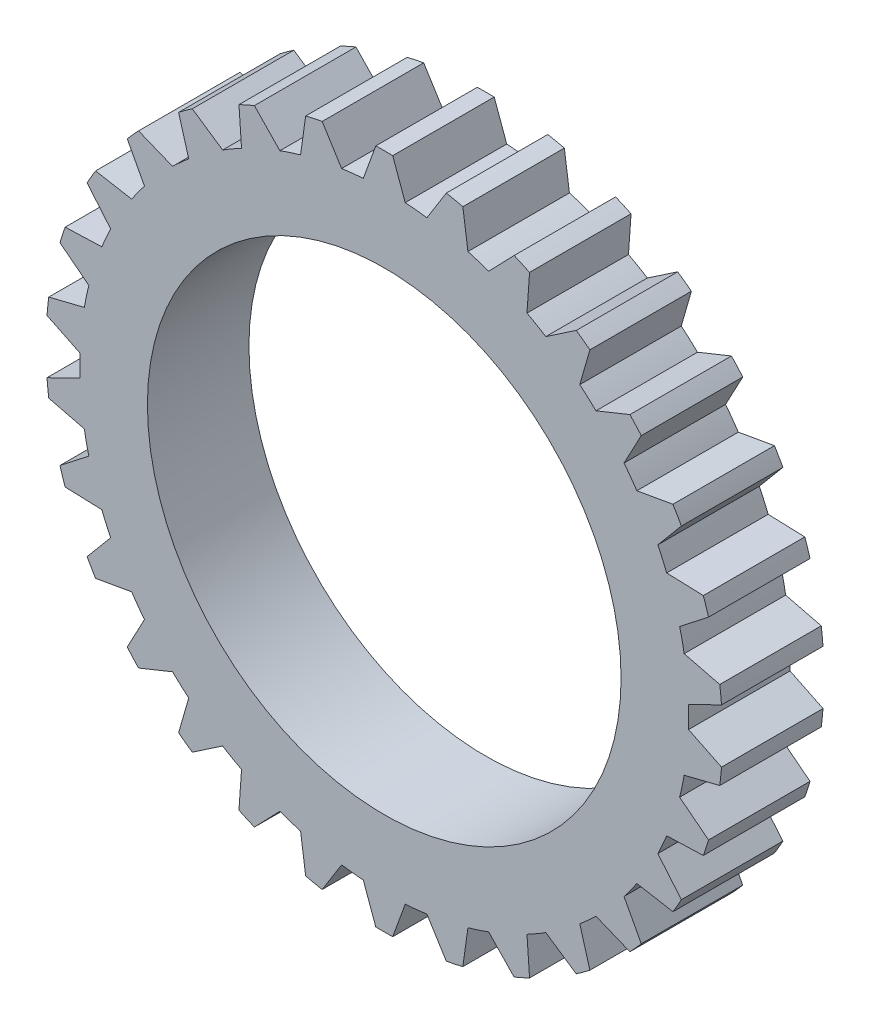
from build123d import *

# Parameters (mm, degrees)
SKETCH1_R           = 70
BOSS_EXTRUDE1_DEPTH = 30


with BuildPart() as part:
    # Sketch1 → Boss-Extrude1 (new body)
    with BuildSketch(Plane.XY):
        with BuildLine():
            Line((-2.5, 99.968745116), (-6.2, 89.786190475))
            ThreePointArc((-6.2, 89.786190475), (-9.407561694, 89.506970583), (-12.603083549, 89.113199275))
            Line((-12.603083549, 89.113199275), (-18.339301824, 98.30396741))
            ThreePointArc((-18.339301824, 98.30396741), (-20.791169082, 97.814760073), (-23.230039828, 97.264408956))
            Line((-23.230039828, 97.264408956), (-24.732113798, 86.535094309))
            ThreePointArc((-24.732113798, 86.535094309), (-27.811529494, 85.595086467), (-30.855351871, 84.545533654))
            Line((-30.855351871, 84.545533654), (-38.377088157, 92.342834614))
            ThreePointArc((-38.377088157, 92.342834614), (-40.673664308, 91.354545764), (-42.944815445, 90.309151399))
            Line((-42.944815445, 90.309151399), (-42.183315546, 79.50199928))
            ThreePointArc((-42.183315546, 79.50199928), (-45, 77.942286341), (-47.759093256, 76.282822519))
            Line((-47.759093256, 76.282822519), (-56.737611583, 82.345876836))
            ThreePointArc((-56.737611583, 82.345876836), (-58.778525229, 80.901699437), (-60.782696555, 79.406950574))
            Line((-60.782696555, 79.406950574), (-57.790903986, 68.99428539))
            ThreePointArc((-57.790903986, 68.99428539), (-60.221754572, 66.883034293), (-62.575533091, 64.686185993))
            Line((-62.575533091, 64.686185993), (-72.618429126, 68.7500091))
            ThreePointArc((-72.618429126, 68.7500091), (-74.314482548, 66.913060636), (-75.964082158, 65.034284972))
            Line((-75.964082158, 65.034284972), (-70.87275261, 55.471190157))
            ThreePointArc((-70.87275261, 55.471190157), (-72.811529494, 52.900672706), (-74.65712186, 50.262452741))
            Line((-74.65712186, 50.262452741), (-85.325472855, 52.149436067))
            ThreePointArc((-85.325472855, 52.149436067), (-86.602540378, 50), (-87.825472855, 47.819309048))
            Line((-87.825472855, 47.819309048), (-80.85712186, 39.523737734))
            ThreePointArc((-80.85712186, 39.523737734), (-82.219091188, 36.606297877), (-83.475836159, 33.642009118))
            Line((-83.475836159, 33.642009118), (-94.303383982, 33.269682438))
            ThreePointArc((-94.303383982, 33.269682438), (-95.10565163, 30.901699437), (-95.848468954, 28.514399856))
            Line((-95.848468954, 28.514399856), (-87.30764689, 21.848908316))
            ThreePointArc((-87.30764689, 21.848908316), (-88.033284066, 18.712052174), (-88.646255857, 15.551248264))
            Line((-88.646255857, 15.551248264), (-99.159784712, 12.93588404))
            ThreePointArc((-99.159784712, 12.93588404), (-99.452189537, 10.452846327), (-99.682427028, 7.963274563))
            Line((-99.682427028, 7.963274563), (-89.942408801, 3.219176762))
            ThreePointArc((-89.942408801, 3.219176762), (-90, 0), (-89.942408801, -3.219176762))
            Line((-89.942408801, -3.219176762), (-99.682427028, -7.963274563))
            ThreePointArc((-99.682427028, -7.963274563), (-99.452189537, -10.452846327), (-99.159784712, -12.93588404))
            Line((-99.159784712, -12.93588404), (-88.646255857, -15.551248264))
            ThreePointArc((-88.646255857, -15.551248264), (-88.033284066, -18.712052174), (-87.30764689, -21.848908316))
            Line((-87.30764689, -21.848908316), (-95.848468954, -28.514399856))
            ThreePointArc((-95.848468954, -28.514399856), (-95.10565163, -30.901699437), (-94.303383982, -33.269682438))
            Line((-94.303383982, -33.269682438), (-83.475836159, -33.642009118))
            ThreePointArc((-83.475836159, -33.642009118), (-82.219091188, -36.606297877), (-80.85712186, -39.523737734))
            Line((-80.85712186, -39.523737734), (-87.825472855, -47.819309048))
            ThreePointArc((-87.825472855, -47.819309048), (-86.602540378, -50), (-85.325472855, -52.149436067))
            Line((-85.325472855, -52.149436067), (-74.65712186, -50.262452741))
            ThreePointArc((-74.65712186, -50.262452741), (-72.811529494, -52.900672706), (-70.87275261, -55.471190157))
            Line((-70.87275261, -55.471190157), (-75.964082158, -65.034284972))
            ThreePointArc((-75.964082158, -65.034284972), (-74.314482548, -66.913060636), (-72.618429126, -68.7500091))
            Line((-72.618429126, -68.7500091), (-62.575533091, -64.686185993))
            ThreePointArc((-62.575533091, -64.686185993), (-60.221754572, -66.883034293), (-57.790903986, -68.99428539))
            Line((-57.790903986, -68.99428539), (-60.782696555, -79.406950574))
            ThreePointArc((-60.782696555, -79.406950574), (-58.778525229, -80.901699437), (-56.737611583, -82.345876836))
            Line((-56.737611583, -82.345876836), (-47.759093256, -76.282822519))
            ThreePointArc((-47.759093256, -76.282822519), (-45, -77.942286341), (-42.183315546, -79.50199928))
            Line((-42.183315546, -79.50199928), (-42.944815445, -90.309151399))
            ThreePointArc((-42.944815445, -90.309151399), (-40.673664308, -91.354545764), (-38.377088157, -92.342834614))
            Line((-38.377088157, -92.342834614), (-30.855351871, -84.545533654))
            ThreePointArc((-30.855351871, -84.545533654), (-27.811529494, -85.595086467), (-24.732113798, -86.535094309))
            Line((-24.732113798, -86.535094309), (-23.230039828, -97.264408956))
            ThreePointArc((-23.230039828, -97.264408956), (-20.791169082, -97.814760073), (-18.339301824, -98.30396741))
            Line((-18.339301824, -98.30396741), (-12.603083549, -89.113199275))
            ThreePointArc((-12.603083549, -89.113199275), (-9.407561694, -89.506970583), (-6.2, -89.786190475))
            Line((-6.2, -89.786190475), (-2.5, -99.968745116))
            ThreePointArc((-2.5, -99.968745116), (0, -100), (2.5, -99.968745116))
            Line((2.5, -99.968745116), (6.2, -89.786190475))
            ThreePointArc((6.2, -89.786190475), (9.407561694, -89.506970583), (12.603083549, -89.113199275))
            Line((12.603083549, -89.113199275), (18.339301824, -98.30396741))
            ThreePointArc((18.339301824, -98.30396741), (20.791169082, -97.814760073), (23.230039828, -97.264408956))
            Line((23.230039828, -97.264408956), (24.732113798, -86.535094309))
            ThreePointArc((24.732113798, -86.535094309), (27.811529494, -85.595086467), (30.855351871, -84.545533654))
            Line((30.855351871, -84.545533654), (38.377088157, -92.342834614))
            ThreePointArc((38.377088157, -92.342834614), (40.673664308, -91.354545764), (42.944815445, -90.309151399))
            Line((42.944815445, -90.309151399), (42.183315546, -79.50199928))
            ThreePointArc((42.183315546, -79.50199928), (45, -77.942286341), (47.759093256, -76.282822519))
            Line((47.759093256, -76.282822519), (56.737611583, -82.345876836))
            ThreePointArc((56.737611583, -82.345876836), (58.778525229, -80.901699437), (60.782696555, -79.406950574))
            Line((60.782696555, -79.406950574), (57.790903986, -68.99428539))
            ThreePointArc((57.790903986, -68.99428539), (60.221754572, -66.883034293), (62.575533091, -64.686185993))
            Line((62.575533091, -64.686185993), (72.618429126, -68.7500091))
            ThreePointArc((72.618429126, -68.7500091), (74.314482548, -66.913060636), (75.964082158, -65.034284972))
            Line((75.964082158, -65.034284972), (70.87275261, -55.471190157))
            ThreePointArc((70.87275261, -55.471190157), (72.811529494, -52.900672706), (74.65712186, -50.262452741))
            Line((74.65712186, -50.262452741), (85.325472855, -52.149436067))
            ThreePointArc((85.325472855, -52.149436067), (86.602540378, -50), (87.825472855, -47.819309048))
            Line((87.825472855, -47.819309048), (80.85712186, -39.523737734))
            ThreePointArc((80.85712186, -39.523737734), (82.219091188, -36.606297877), (83.475836159, -33.642009118))
            Line((83.475836159, -33.642009118), (94.303383982, -33.269682438))
            ThreePointArc((94.303383982, -33.269682438), (95.10565163, -30.901699437), (95.848468954, -28.514399856))
            Line((95.848468954, -28.514399856), (87.30764689, -21.848908316))
            ThreePointArc((87.30764689, -21.848908316), (88.033284066, -18.712052174), (88.646255857, -15.551248264))
            Line((88.646255857, -15.551248264), (99.159784712, -12.93588404))
            ThreePointArc((99.159784712, -12.93588404), (99.452189537, -10.452846327), (99.682427028, -7.963274563))
            Line((99.682427028, -7.963274563), (89.942408801, -3.219176762))
            ThreePointArc((89.942408801, -3.219176762), (90, 0), (89.942408801, 3.219176762))
            Line((89.942408801, 3.219176762), (99.682427028, 7.963274563))
            ThreePointArc((99.682427028, 7.963274563), (99.452189537, 10.452846327), (99.159784712, 12.93588404))
            Line((99.159784712, 12.93588404), (88.646255857, 15.551248264))
            ThreePointArc((88.646255857, 15.551248264), (88.033284066, 18.712052174), (87.30764689, 21.848908316))
            Line((87.30764689, 21.848908316), (95.848468954, 28.514399856))
            ThreePointArc((95.848468954, 28.514399856), (95.10565163, 30.901699437), (94.303383982, 33.269682438))
            Line((94.303383982, 33.269682438), (83.475836159, 33.642009118))
            ThreePointArc((83.475836159, 33.642009118), (82.219091188, 36.606297877), (80.85712186, 39.523737734))
            Line((80.85712186, 39.523737734), (87.825472855, 47.819309048))
            ThreePointArc((87.825472855, 47.819309048), (86.602540378, 50), (85.325472855, 52.149436067))
            Line((85.325472855, 52.149436067), (74.65712186, 50.262452741))
            ThreePointArc((74.65712186, 50.262452741), (72.811529494, 52.900672706), (70.87275261, 55.471190157))
            Line((70.87275261, 55.471190157), (75.964082158, 65.034284972))
            ThreePointArc((75.964082158, 65.034284972), (74.314482548, 66.913060636), (72.618429126, 68.7500091))
            Line((72.618429126, 68.7500091), (62.575533091, 64.686185993))
            ThreePointArc((62.575533091, 64.686185993), (60.221754572, 66.883034293), (57.790903986, 68.99428539))
            Line((57.790903986, 68.99428539), (60.782696555, 79.406950574))
            ThreePointArc((60.782696555, 79.406950574), (58.778525229, 80.901699437), (56.737611583, 82.345876836))
            Line((56.737611583, 82.345876836), (47.759093256, 76.282822519))
            ThreePointArc((47.759093256, 76.282822519), (45, 77.942286341), (42.183315546, 79.50199928))
            Line((42.183315546, 79.50199928), (42.944815445, 90.309151399))
            ThreePointArc((42.944815445, 90.309151399), (40.673664308, 91.354545764), (38.377088157, 92.342834614))
            Line((38.377088157, 92.342834614), (30.855351871, 84.545533654))
            ThreePointArc((30.855351871, 84.545533654), (27.811529494, 85.595086467), (24.732113798, 86.535094309))
            Line((24.732113798, 86.535094309), (23.230039828, 97.264408956))
            ThreePointArc((23.230039828, 97.264408956), (20.791169082, 97.814760073), (18.339301824, 98.30396741))
            Line((18.339301824, 98.30396741), (12.603083549, 89.113199275))
            ThreePointArc((12.603083549, 89.113199275), (9.407561694, 89.506970583), (6.2, 89.786190475))
            Line((6.2, 89.786190475), (2.5, 99.968745116))
            ThreePointArc((2.5, 99.968745116), (0, 100), (-2.5, 99.968745116))
        make_face()
        Circle(SKETCH1_R, mode=Mode.SUBTRACT)
    extrude(amount=BOSS_EXTRUDE1_DEPTH)


solid = part.part
